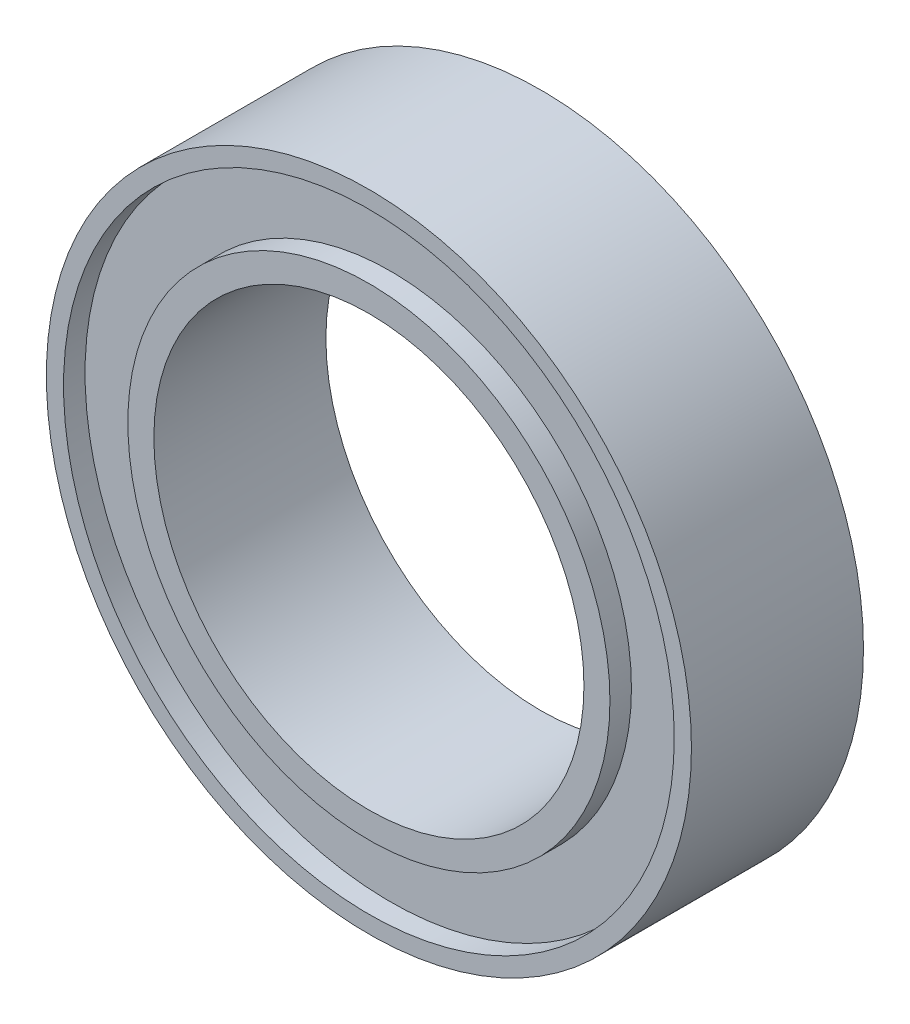
from build123d import *

# Parameters (mm, degrees)
BOSS_EXTRUDE1_DEPTH      = 2
BOSS_EXTRUDE1_DEPTH_BACK = 2
SKETCH1_R                = 7.5
SKETCH1_R_2              = 5
SKETCH2_R                = 7.1
SKETCH2_R_2              = 5.605
CUT_EXTRUDE1_DEPTH       = 0.5


with BuildPart() as part:
    # Sketch1 → Boss-Extrude1 (new, two sides: drawn at the far end of the back side and taken through both)
    with BuildSketch(Plane.XY.offset(-BOSS_EXTRUDE1_DEPTH_BACK)):
        Circle(SKETCH1_R)
        Circle(SKETCH1_R_2, mode=Mode.SUBTRACT)
    extrude(amount=BOSS_EXTRUDE1_DEPTH + BOSS_EXTRUDE1_DEPTH_BACK)

    # Sketch2 → Cut-Extrude1 (cut)
    with BuildSketch(Plane.XY.offset(2)):
        Circle(SKETCH2_R)
        Circle(SKETCH2_R_2, mode=Mode.SUBTRACT)
    cut_extrude1 = extrude(amount=-CUT_EXTRUDE1_DEPTH, mode=Mode.SUBTRACT)

    # Mirror1: Cut-Extrude1 across plane
    add(cut_extrude1.mirror(Plane.XY), mode=Mode.SUBTRACT)


solid = part.part
